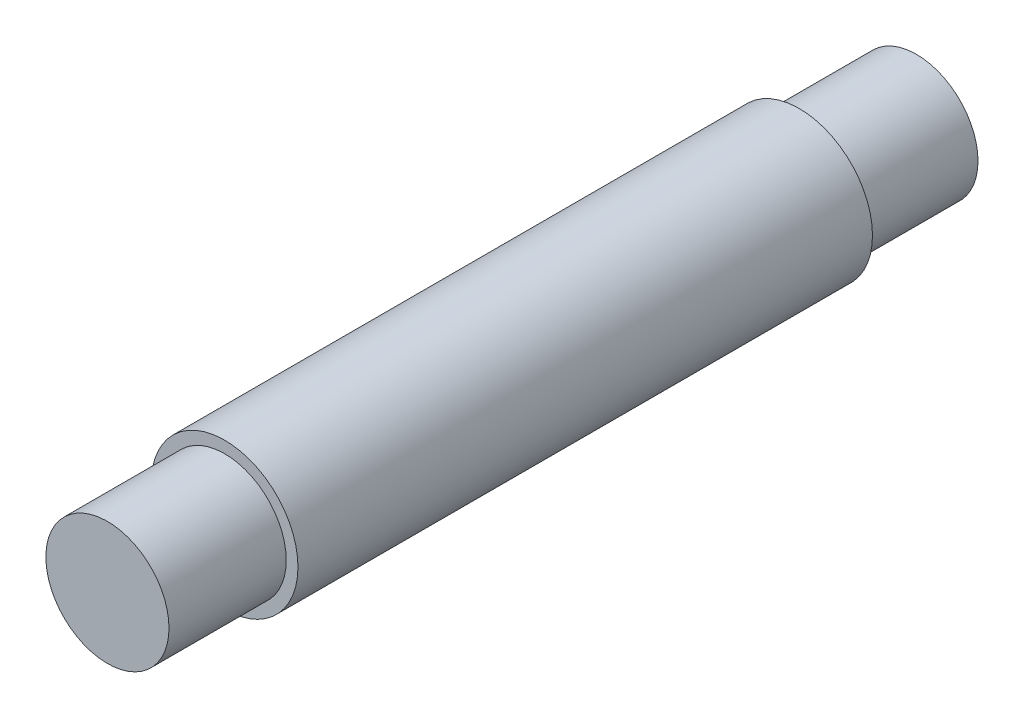
from build123d import *

# Parameters (mm, degrees)
SKETCH_1_R           = 25
BOSS_EXTRUDE_1_DEPTH = 98
SKETCH_2_R           = 21
BOSS_EXTRUDE_2_DEPTH = 40


with BuildPart() as part:
    # Sketch 1 → Boss-Extrude 1 (new, symmetric)
    with BuildSketch(Plane.XY):
        Circle(SKETCH_1_R)
    extrude(amount=BOSS_EXTRUDE_1_DEPTH, both=True)

    # Sketch 2 → Boss-Extrude 2 (add)
    with BuildSketch(Plane.XY.offset(98)):
        Circle(SKETCH_2_R)
    boss_extrude_2 = extrude(amount=BOSS_EXTRUDE_2_DEPTH)

    # Mirror 1: Boss-Extrude 2 across plane
    add(boss_extrude_2.mirror(Plane.XY))


solid = part.part
